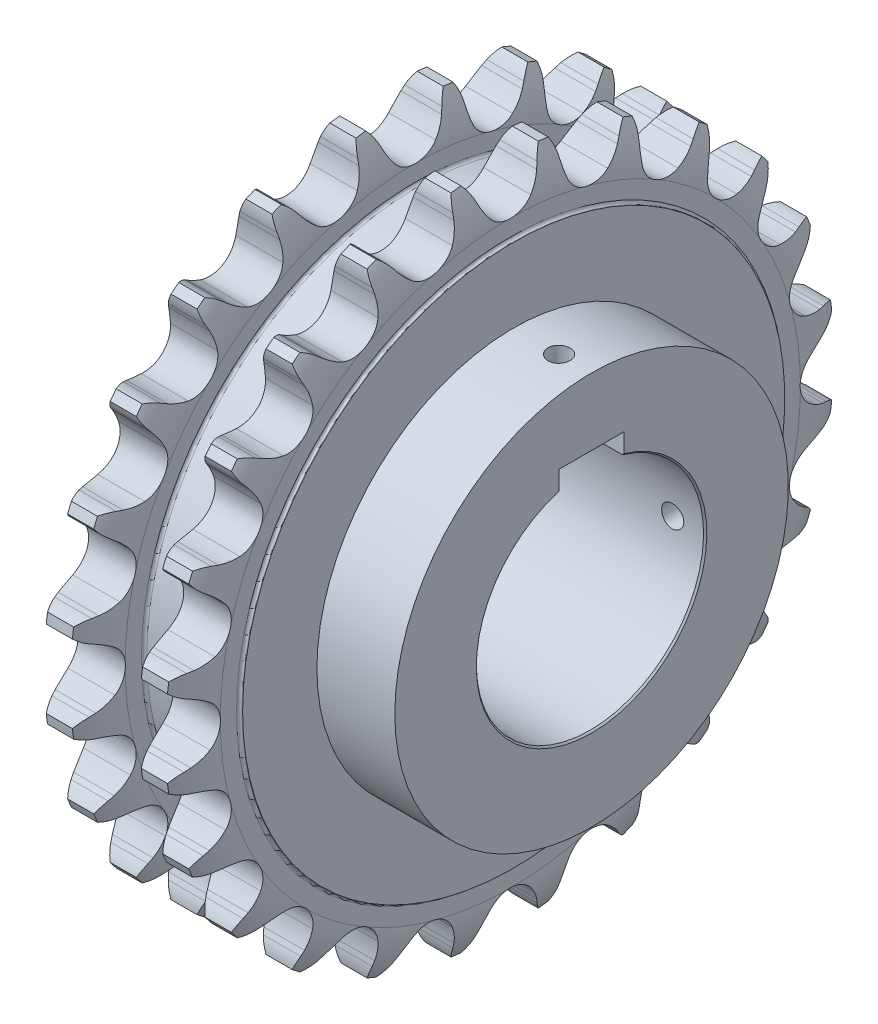
SolidWorks part; units mm, degrees
ref_plane "Front Plane" through (0, 0, 0) normal (0, 0, 1) x (1, 0, 0)
ref_plane "Top Plane" through (0, 0, 0) normal (0, 1, 0) x (1, 0, 0)
ref_plane "Right Plane" through (0, 0, 0) normal (1, 0, 0) x (0, 0, -1)
sketch "Sketch1" plane through (0, 0, 0) normal (0, 0, 1) x (1, 0, 0)
  line L0 (-12.7, 0) -> (12.7, 0) construction
  line L1 (-8.3587, 35) -> (-8.3587, 83.5)
  line L2 (-8.3587, 83.5) -> (-8.1517, 83.5)
  line L3 (-7.3237, 84.3279) -> (-7.3237, 89.3585)
  line L4 (-4.0217, 103) -> (4.0217, 103)
  line L5 (7.3237, 89.3585) -> (7.3237, 84.3279)
  line L6 (8.1517, 83.5) -> (8.3587, 83.5)
  line L7 (8.3587, 83.5) -> (8.3587, 35)
  line L8 (8.3587, 35) -> (-8.3587, 35)
  line L9 (0, 0) -> (0, 103) construction
  line L10 (-6.4021, 97.2985) -> (6.4021, 97.2985) construction
  line L11 (-6.4021, -97.2985) -> (6.4021, -97.2985) construction
  line L12 (12.7, 0) -> (36.7, 0) construction
  line L13 (-7.3237, 89.3585) -> (3.7984, 89.3585) construction
  line L14 (-7.3237, -89.3585) -> (3.7984, -89.3585) construction
  line L15 (36.7, 0) -> (52.58, 0) construction
  line L16 (52.58, 0) -> (76.71, 0) construction
  line L17 (76.71, 0) -> (92.46, 0) construction
  line L18 (92.46, 0) -> (121.75, 0) construction
  arc A0 (-4.0217, 103) -> (-7.3237, 89.3585) centre (18.0534, 90.4362) ccw
  arc A1 (4.0217, 103) -> (7.3237, 89.3585) centre (-18.0534, 90.4362) cw
  arc A2 (7.3237, 84.3279) -> (8.1517, 83.5) centre (8.1517, 84.3279) ccw
  arc A3 (-8.1517, 83.5) -> (-7.3237, 84.3279) centre (-8.1517, 84.3279) ccw
  point P30 (7.3237, 83.5)
  point P33 (-7.3237, 83.5)
  dimension "rx" = 25.4
  dimension "D3" = 0.8279
  dimension "d" = 194.597
  dimension "p" = 25.4
  dimension "z" = 24
  dimension "da" = 206
  dimension "df" = 178.717
  dimension "dr" = 15.88
  dimension "dk" = 70
  dimension "dg" = 167
  dimension "h" = 24.13
  dimension "bf1" = 14.6475
  dimension "b1" = 15.75
  dimension "ba" = 3.302
  dimension "D2" = 1.0349
  dimension "pt" = 29.29
revolve "Revolve1" add sketch "Sketch1" angle 360 about L0
sketch "Sketch2" plane through (0, 0, 0) normal (1, 0, 0) x (0, 0, -1)
  line L0 (0, 0) -> (0, 103) construction
  line L1 (0, 0) -> (-13.4442, 102.1188) construction
  line L2 (0, 0) -> (-26.6584, 99.4904) construction
  line L3 (6.3704, 92.4103) -> (31.4819, 73.1415) construction
  line L4 (9.1677, 97.3212) -> (-10.0788, 105.0322) construction
  line L5 (0, 0) -> (13.4442, 102.1188) construction
  line L6 (9.1677, 97.3212) -> (9.7925, 98.8807)
  line L7 (-9.1677, 97.3212) -> (-9.7925, 98.8807)
  circle A0 centre (0, 0) radius 103 construction
  arc A1 (6.3704, 92.4103) -> (-6.3704, 92.4103) centre (0, 97.2985) cw
  arc A2 (6.3704, 92.4103) -> (9.1677, 97.3212) centre (-10.0788, 105.0322) ccw
  arc A3 (11.9288, 102.3069) -> (9.7925, 98.8807) centre (20.4674, 94.6039) ccw
  arc A4 (-6.3704, 92.4103) -> (-9.1677, 97.3212) centre (10.0788, 105.0322) cw
  arc A5 (-11.9288, 102.3069) -> (-9.7925, 98.8807) centre (-20.4674, 94.6039) cw
  arc A7 (11.9288, 102.3069) -> (-11.9288, 102.3069) centre (0, 0) ccw
  dimension "r1" = 8.0297
  dimension "r3" = 11.4997
  dimension "D1" = 15
  dimension "D2" = 7.5
  dimension "α/2" = 52.5
  dimension "M" = 10.0788
  dimension "T" = 7.7337
  dimension "β" = 15.667
  dimension "γ/2" = 14.333
  dimension "bc" = 1.6801
extrude "Cut-Extrude1" cut sketch "Sketch2" against normal mid plane 16.7173
pattern_circular "CirPattern1" count 24 over 360 about axis through (0, 0, 0) along (1, 0, 0) of "Cut-Extrude1"
pattern_linear "LPattern1" count 2 spacing 29.29 along (1, 0, 0) of bodies 103
sketch "Sketch7" plane through (0, 0, 0) normal (0, 0, 1) x (1, 0, 0)
  line L0 (0, 0) -> (14.4569, 0) construction
  line L1 (8.3587, 35) -> (36.8207, 35)
  line L2 (8.3587, 35) -> (8.3587, 83.5)
  line L3 (8.3587, 83.5) -> (36.8207, 83.5)
  line L4 (36.8207, 35) -> (36.8207, 83.5)
  dimension "L" = 44.9724
revolve "Revolve4" add sketch "Sketch7" angle 360 about L0
sketch "Sketch3" plane through (0, 0, 0) normal (0, 0, 1) x (1, 0, 0)
  line L0 (8.3587, 35) -> (61.6413, 35)
  line L3 (61.6413, 35) -> (61.6413, 60.6126)
  line L4 (61.6413, 60.6126) -> (8.3587, 60.6126)
  line L5 (8.3587, 60.6126) -> (8.3587, 35)
  line L6 (0, 0) -> (9.5, 0) construction
  line L8 (-8.3587, 83.5) -> (-8.3587, -83.5) construction
  dimension "h" = 25.6126
  dimension "K" = 9.5
  dimension "L" = 70
revolve "Revolve2" add sketch "Sketch3" angle 360 about L6
sketch "Sketch4" plane through (-8.3587, 0, 0) normal (-1, 0, 0) x (0, 0, 1)
  line L0 (0, 35) -> (0, 39.9) construction
  line L1 (-10, 33.541) -> (10, 33.541)
  line L2 (-10, 33.541) -> (-10, 39.9)
  line L3 (-10, 39.9) -> (10, 39.9)
  line L4 (10, 33.541) -> (10, 39.9)
  circle A0 centre (0, 0) radius 35 construction
  point P6 (4.6, 39.9)
  dimension "D1" = 4.9
  dimension "键槽宽度" = 20
  dimension "t1" = 5.4
extrude "Cut-Extrude2" cut sketch "Sketch4" against normal through all
chamfer "Chamfer1" distance 1 angle 45 1 edges at (-8.3587, -35, 0)
chamfer "Chamfer3" distance 0.5 angle 45 1 edges at (61.6413, -35, 0)
ref_plane "Plane1" through (0, 0, -60.6126) normal (0, 0, -1) x (-1, 0, 0)
sketch "Sketch8" plane through (0, 0, -60.6126) normal (0, 0, -1) x (-1, 0, 0)
  line L0 (-61.6413, 0) -> (8.1517, 0) construction
  line L1 (-61.6413, 60.6126) -> (-61.6413, -60.6126) construction
  line L2 (8.1517, 83.5) -> (8.1517, -83.5) construction
  circle A0 centre (-51.6413, 0) radius 3.4
  dimension "D1" = 6.8
  dimension "D2" = 10
extrude "Cut-Extrude3" cut sketch "Sketch8" against normal blind 30
ref_plane "Plane2" through (0, 60.6126, 0) normal (0, 1, 0) x (1, 0, 0)
sketch "Sketch9" plane through (0, 60.6126, 0) normal (0, 1, 0) x (1, 0, 0)
  line L0 (61.6413, -60.6126) -> (61.6413, 60.6126) construction
  line L1 (61.6413, 0) -> (-8.1517, 0) construction
  line L2 (-8.1517, -83.5) -> (-8.1517, 83.5) construction
  circle A0 centre (51.6413, 0) radius 3.4
  dimension "D2" = 6.8
  dimension "D1" = 10
extrude "Cut-Extrude4" cut sketch "Sketch9" against normal blind 30
hole_wizard "Tap Drill for M10 Tap1" positions "Sketch12" profile "Sketch14" hole size "M10" standard "GB"
sketch "Sketch12" plane through (-8.3587, 0, 0) normal (-1, 0, 0) x (0, 0, 1)
  circle A0 centre (0, 0) radius 60 construction
  point P0 (0, 60)
  point P8 (-60, 0)
  point P10 (0, -60)
  point P12 (60, 0)
  dimension "D1" = 120
sketch "Sketch14" plane through (-8.3587, 60, 0) normal (0, 1, 0) x (0, 0, 1)
  line L0 (0, 0) -> (0, 22.5537)
  line L1 (0, 22.5537) -> (4.25, 20)
  line L2 (4.25, 20) -> (4.25, 0)
  line L5 (4.25, 0) -> (0, 0)
  line L10 (0, 22.5537) -> (-4.25, 20) construction
  line L11 (0, -6.35) -> (0, 107.95) construction
  dimension "孔直径" = 8.5
  dimension "孔深度" = 20
  dimension "导头角度" = 118
ref_plane "Plane3" through (14.645, 0, 0) normal (1, 0, 0) x (0, 0, -1)
